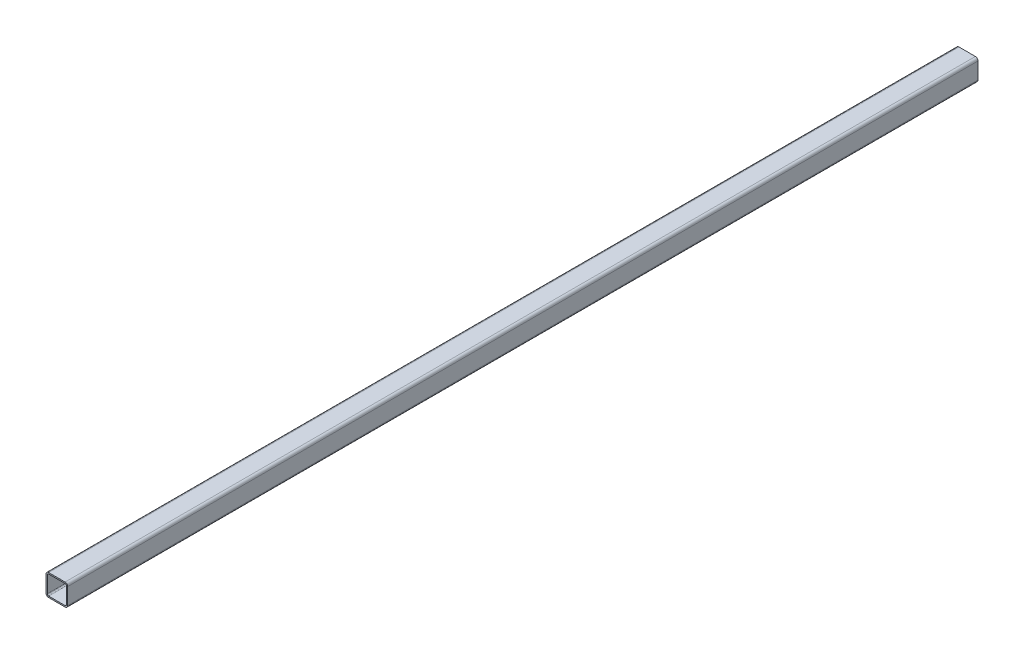
from build123d import *

# Parameters (mm, degrees)
GB_6728_1986_050_X_50_X_3_1_DEPTH = 2100


with BuildPart() as part:
    # Sketch1 → Gb／6728-1986方形空心型钢 050 X 50 X 3(1) (new body)
    with BuildSketch(Plane.YX.offset(-1050)):
        with BuildLine():
            Line((-19, -25), (19, -25))
            ThreePointArc((19, -25), (23.242640687, -23.242640687), (25, -19))
            Line((25, -19), (25, 19))
            ThreePointArc((25, 19), (23.242640687, 23.242640687), (19, 25))
            Line((19, 25), (-19, 25))
            ThreePointArc((-19, 25), (-23.242640687, 23.242640687), (-25, 19))
            Line((-25, 19), (-25, -19))
            ThreePointArc((-25, -19), (-23.242640687, -23.242640687), (-19, -25))
        make_face()
        with BuildLine():
            Line((-19, -22), (19, -22))
            ThreePointArc((19, -22), (21.121320344, -21.121320344), (22, -19))
            Line((22, -19), (22, 19))
            ThreePointArc((22, 19), (21.121320344, 21.121320344), (19, 22))
            Line((19, 22), (-19, 22))
            ThreePointArc((-19, 22), (-21.121320344, 21.121320344), (-22, 19))
            Line((-22, 19), (-22, -19))
            ThreePointArc((-22, -19), (-21.121320344, -21.121320344), (-19, -22))
        make_face(mode=Mode.SUBTRACT)
    extrude(amount=GB_6728_1986_050_X_50_X_3_1_DEPTH)


solid = part.part
